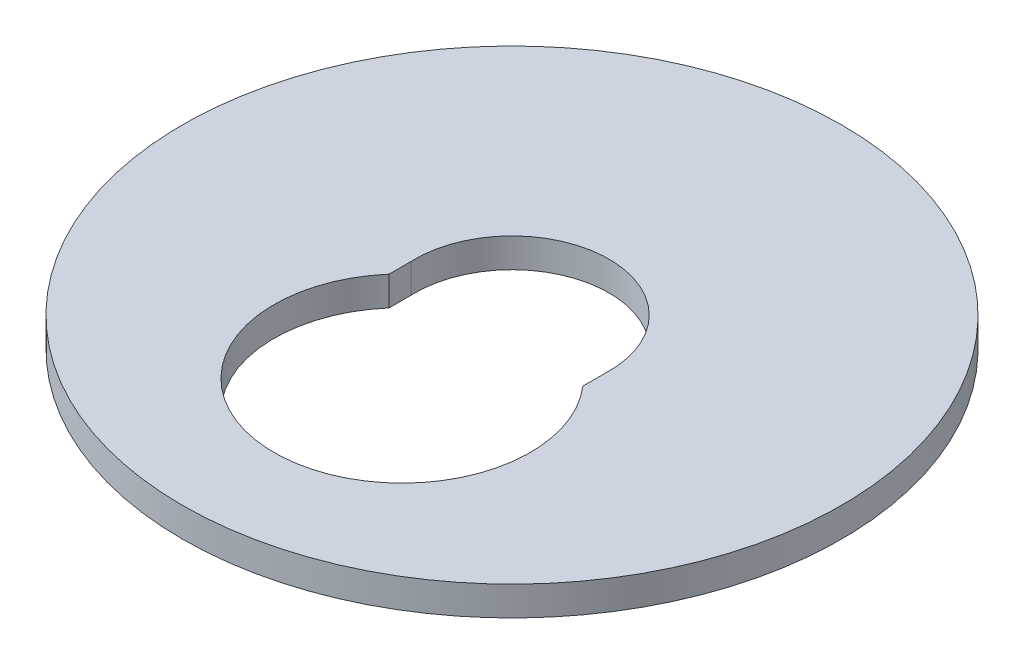
from build123d import *

# Parameters (mm, degrees)
SKETCH_1_R          = 45
SKETCH_1_R_2        = 13.25
EXTRUDE_1_DEPTH     = 2
CUT_EXTRUDE_1_REACH = 65.765


with BuildPart() as part:
    # 草图1 → 凸台-拉伸1 (new, symmetric)
    with BuildSketch(Plane(origin=(0, 0, 0), x_dir=(1, 0, 0), z_dir=(0, 1, 0))):
        with Locations(Location((0, 0, 0), (0, 0, 270))):
            Circle(SKETCH_1_R)
        with Locations(Location((0, 0, 0), (0, 0, 270))):
            Circle(SKETCH_1_R_2, mode=Mode.SUBTRACT)
    extrude(amount=EXTRUDE_1_DEPTH, both=True)

    # 草图2 → 切除-拉伸1 (cut, up to next)
    with BuildSketch(Plane.XZ.offset(2), mode=Mode.PRIVATE) as cut_extrude_1_sk1:
        with BuildLine():
            Line((-13.23838441, 0.5546875), (-13.23838441, 3.5546875))
            ThreePointArc((-13.23838441, 3.5546875), (0, 32.5), (13.23838441, 3.5546875))
            Line((13.23838441, 3.5546875), (13.23838441, 0.5546875))
            Line((13.23838441, 0.5546875), (-13.23838441, 0.5546875))
        make_face()
    cut_extrude_1_tool1 = extrude(cut_extrude_1_sk1.sketch, amount=-CUT_EXTRUDE_1_REACH, mode=Mode.PRIVATE) & part.part
    add(cut_extrude_1_tool1.solids().sort_by_distance((0, -2, 15.557308))[0], mode=Mode.SUBTRACT)


solid = part.part
